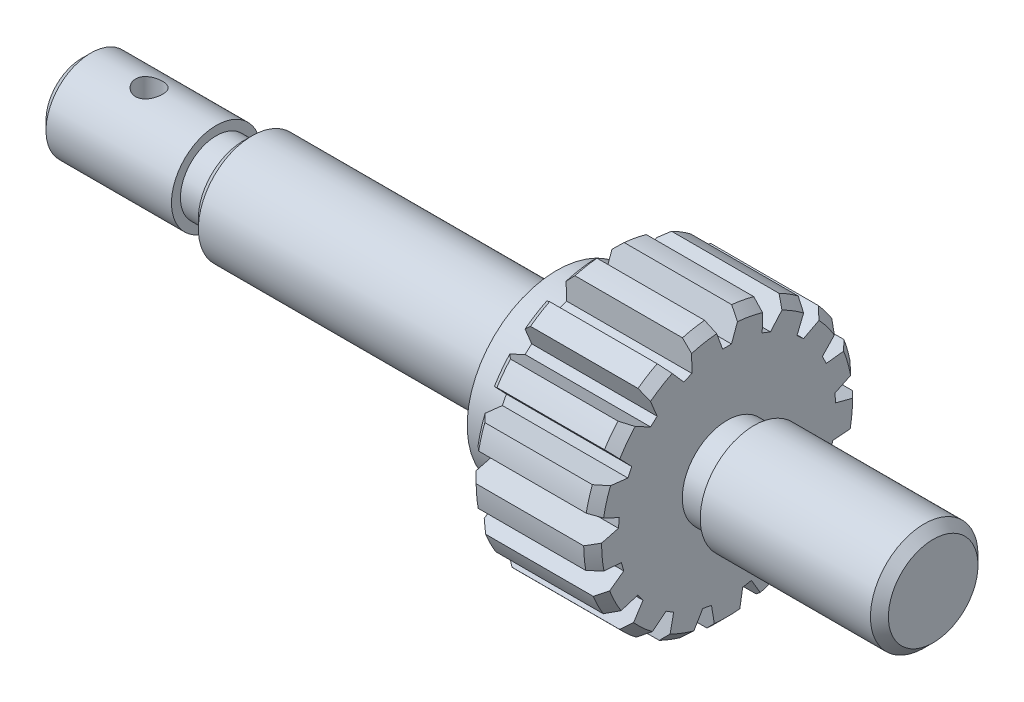
from build123d import *

# Parameters (mm, degrees)
SKETCH1_R            = 5
BOSS_EXTRUDE1_DEPTH  = 15
SKETCH2_R            = 4
BOSS_EXTRUDE2_DEPTH  = 3
SKETCH3_R            = 6
BOSS_EXTRUDE3_DEPTH  = 35
SKETCH4_R            = 10
BOSS_EXTRUDE4_DEPTH  = 5
SKETCH5_R            = 15
BOSS_EXTRUDE5_DEPTH  = 14
SKETCH6_R            = 5
BOSS_EXTRUDE6_DEPTH  = 3
SKETCH7_R            = 6
BOSS_EXTRUDE7_DEPTH  = 20
CHAMFER1_SIZE        = 1
CUT_EXTRUDE1_DEPTH   = 62.757590627
CIRPATTERN1_COUNT    = 17
CUT_SWEEP1_PROFILE_R = 1.5


with BuildPart() as part:
    # Sketch1 → Boss-Extrude1 (new body)
    with BuildSketch(Plane(origin=(0, 0, 0), x_dir=(0, 0, -1), z_dir=(1, 0, 0))):
        Circle(SKETCH1_R)
    extrude(amount=BOSS_EXTRUDE1_DEPTH)

    # Sketch2 → Boss-Extrude2 (add)
    with BuildSketch(Plane(origin=(15, 0, 0), x_dir=(0, 0, -1), z_dir=(1, 0, 0))):
        Circle(SKETCH2_R)
    extrude(amount=BOSS_EXTRUDE2_DEPTH)

    # Sketch3 → Boss-Extrude3 (add)
    with BuildSketch(Plane(origin=(18, 0, 0), x_dir=(0, 0, -1), z_dir=(1, 0, 0))):
        Circle(SKETCH3_R)
    extrude(amount=BOSS_EXTRUDE3_DEPTH)

    # Sketch4 → Boss-Extrude4 (add)
    with BuildSketch(Plane(origin=(53, 0, 0), x_dir=(0, 0, -1), z_dir=(1, 0, 0))):
        Circle(SKETCH4_R)
    extrude(amount=BOSS_EXTRUDE4_DEPTH)

    # Sketch5 → Boss-Extrude5 (add)
    with BuildSketch(Plane(origin=(58, 0, 0), x_dir=(0, 0, -1), z_dir=(1, 0, 0))):
        Circle(SKETCH5_R)
    extrude(amount=BOSS_EXTRUDE5_DEPTH)

    # Sketch6 → Boss-Extrude6 (add)
    with BuildSketch(Plane(origin=(72, 0, 0), x_dir=(0, 0, -1), z_dir=(1, 0, 0))):
        Circle(SKETCH6_R)
    extrude(amount=BOSS_EXTRUDE6_DEPTH)

    # Sketch7 → Boss-Extrude7 (add)
    with BuildSketch(Plane(origin=(75, 0, 0), x_dir=(0, 0, -1), z_dir=(1, 0, 0))):
        Circle(SKETCH7_R)
    extrude(amount=BOSS_EXTRUDE7_DEPTH)

    # Chamfer1
    chamfer1_edges = [part.edges().sort_by_distance(p)[0] for p in [
        (18, 0, 6),
        (58, 0, 15),
        (72, 0, 15),
        (0, 0, 5),
        (95, 0, 6),
    ]]
    chamfer(chamfer1_edges, length=CHAMFER1_SIZE)

    # Sketch8 → Cut-Extrude1 (cut, symmetric)
    with BuildSketch(Plane.ZY.offset(-58)):
        Polygon((2.175583012, 16.742210538), (-2.175583012, 16.742210538), (-0.495055811, 12.125), (0.495055811, 12.125), align=None)
    cut_extrude1 = extrude(amount=CUT_EXTRUDE1_DEPTH, both=True, mode=Mode.SUBTRACT)

    # CirPattern1: Cut-Extrude1 ×17 about axis
    cirpattern1_axis = Axis((0, 0, 0), (1, 0, 0))
    for i in range(1, CIRPATTERN1_COUNT):
        add(cut_extrude1.rotate(cirpattern1_axis, i * 360 / CIRPATTERN1_COUNT), mode=Mode.SUBTRACT)

    # Cut-Sweep1: sweep along a path in Sketch9
    with BuildLine(Plane.XY) as cut_sweep1_path:
        Line((7.5, 10.172757983), (7.5, -6.529018922))
    # Cut-Sweep1 profile (on start of the path) → Cut-Sweep1 (sweep, cut)
    with BuildSketch(Plane(origin=(7.5, 10.172757983, 0), x_dir=(-1, 0, 0), z_dir=(0, -1, 0))):
        Circle(CUT_SWEEP1_PROFILE_R)
    sweep(path=cut_sweep1_path.line, mode=Mode.SUBTRACT)


solid = part.part
